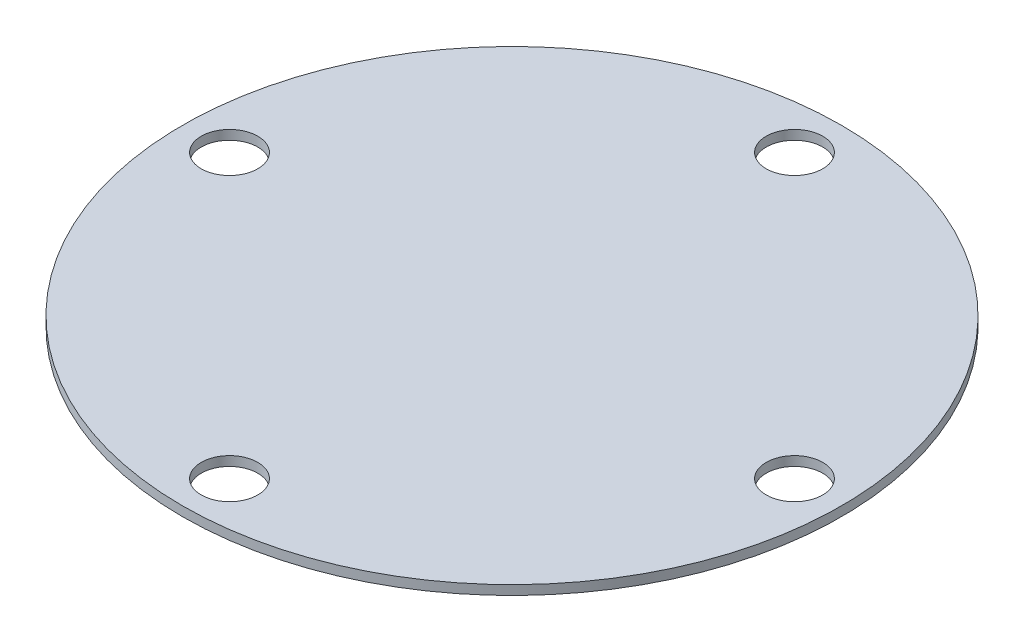
SolidWorks part; units mm, degrees
material "耐油橡胶Ⅰ- 2"
ref_plane "前视基准面" through (0, 0, 0) normal (0, 0, 1) x (1, 0, 0)
ref_plane "上视基准面" through (0, 0, 0) normal (0, 1, 0) x (1, 0, 0)
ref_plane "右视基准面" through (0, 0, 0) normal (1, 0, 0) x (0, 0, -1)
sketch "草图1" plane through (0, 0, 0) normal (0, 1, 0) x (1, 0, 0)
  circle A0 centre (0, 0) radius 70
  dimension "D1" = 140
extrude "凸台-拉伸1" add sketch "草图1" along normal blind 2
sketch "草图3" plane through (0, 2, 0) normal (0, 1, 0) x (1, 0, 0)
  circle A0 centre (0, 0) radius 60 construction
  circle A1 centre (0, 60) radius 6
  circle A2 centre (60, 0) radius 6
  circle A3 centre (0, -60) radius 6
  circle A4 centre (-60, 0) radius 6
  point P14 (0, 0)
  dimension "D1" = 120
  dimension "D2" = 12
  dimension "D3" = 4
extrude "切除-拉伸1" cut sketch "草图3" against normal through all
